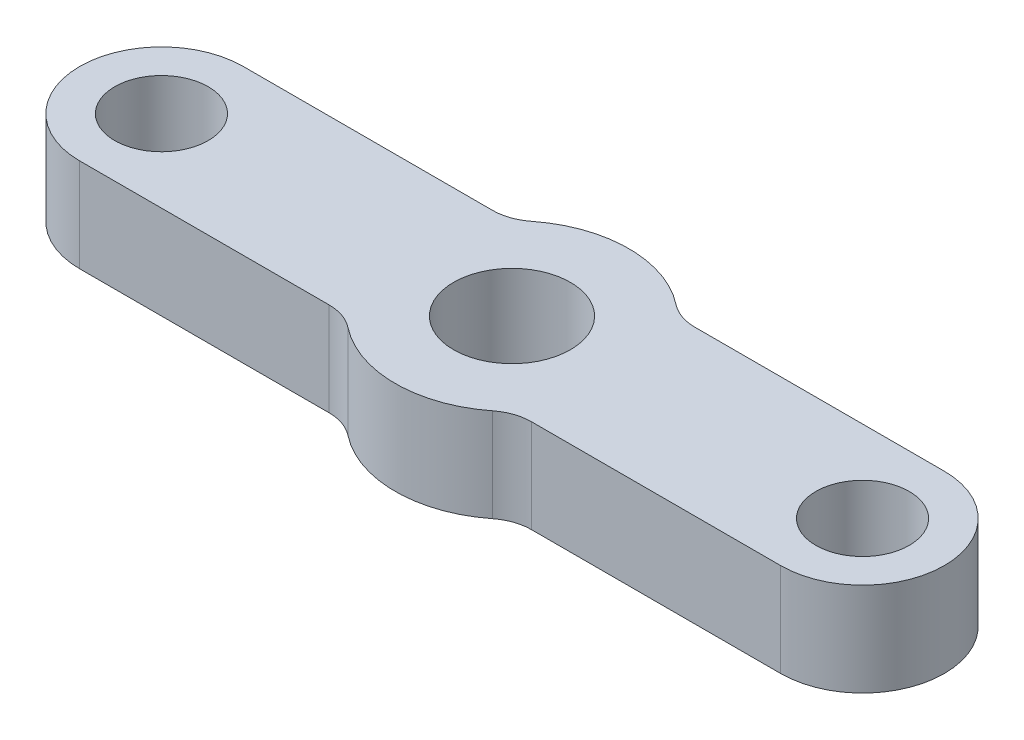
SolidWorks part; units mm, degrees
material "1060 Alloy"
ref_plane "Front Plane" through (0, 0, 0) normal (0, 0, 1) x (1, 0, 0)
ref_plane "Top Plane" through (0, 0, 0) normal (0, 1, 0) x (1, 0, 0)
ref_plane "Right Plane" through (0, 0, 0) normal (1, 0, 0) x (0, 0, -1)
sketch "Sketch1" plane through (0, 0, 0) normal (0, 1, 0) x (1, 0, 0)
  line L0 (0, 28.6415) -> (0, -35.6353) construction
  line L1 (30, 7) -> (8.6603, 7)
  line L2 (30, -7) -> (8.6603, -7)
  line L3 (-30, 7) -> (-8.6603, 7)
  line L4 (-30, -7) -> (-8.6603, -7)
  circle A0 centre (0, 0) radius 5
  arc A1 (6.1859, 7.8571) -> (-6.1859, 7.8571) centre (0, 0) ccw
  circle A2 centre (30, 0) radius 4
  arc A3 (30, -7) -> (30, 7) centre (30, 0) ccw
  arc A4 (8.6603, -7) -> (6.1859, -7.8571) centre (8.6603, -11) ccw
  arc A5 (8.6603, 7) -> (6.1859, 7.8571) centre (8.6603, 11) cw
  circle A6 centre (-30, 0) radius 4
  arc A7 (-30, -7) -> (-30, 7) centre (-30, 0) cw
  arc A8 (-8.6603, -7) -> (-6.1859, -7.8571) centre (-8.6603, -11) cw
  arc A9 (-8.6603, 7) -> (-6.1859, 7.8571) centre (-8.6603, 11) ccw
  arc A10 (-6.1859, -7.8571) -> (6.1859, -7.8571) centre (0, 0) ccw
  dimension "D1" = 10
  dimension "D2" = 20
  dimension "D3" = 8
  dimension "D4" = 14
  dimension "D6" = 4
  dimension "D5" = 30
extrude "Boss-Extrude1" add sketch "Sketch1" along normal blind 8
scale "Scale1" scale about origin uniform scaling yes scale factor 0.5
